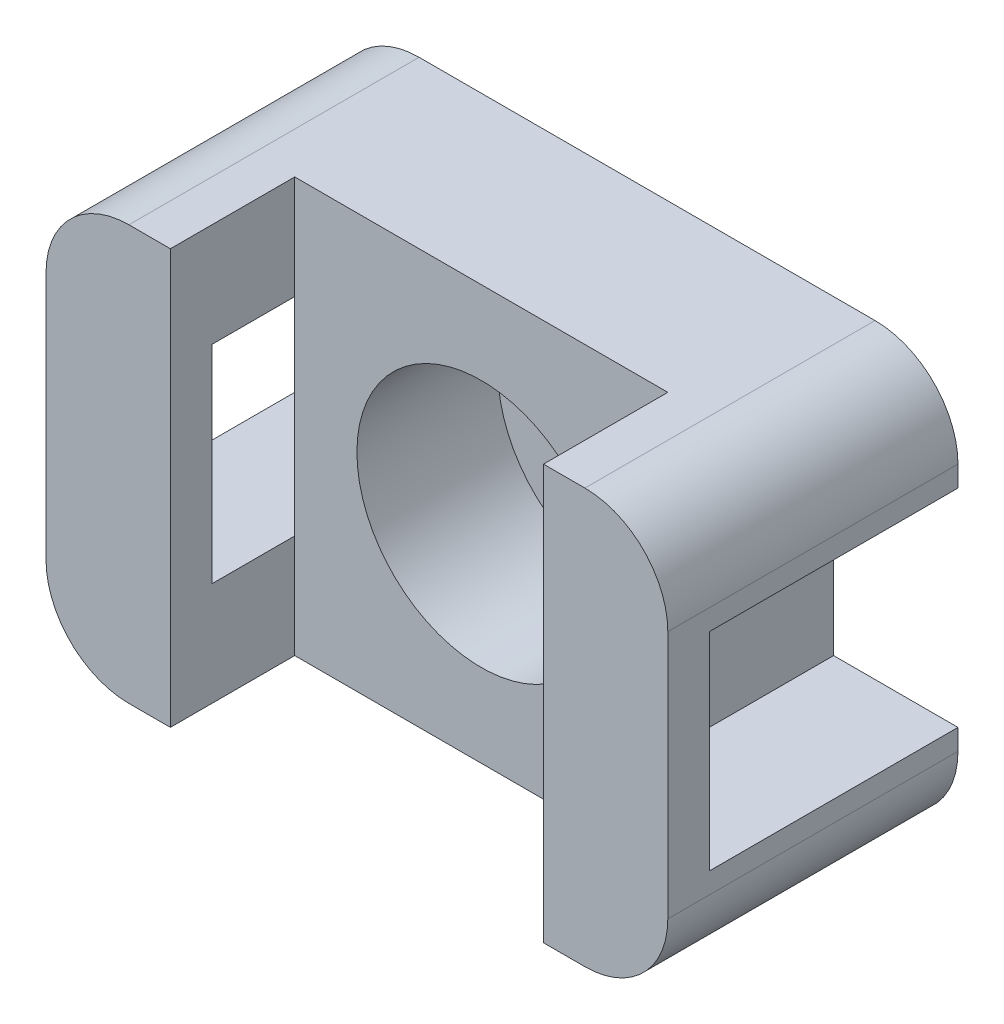
from build123d import *

# Parameters (mm, degrees)
SKETCH1_W                                            = 15
SKETCH1_H                                            = 10
BOSS_EXTRUDE1_DEPTH                                  = 7
SKETCH2_W                                            = 9
SKETCH2_H                                            = 15.767491366
CUT_EXTRUDE1_DEPTH                                   = 3
SKETCH4_W                                            = 6
SKETCH4_H                                            = 5
CUT_EXTRUDE3_DEPTH                                   = 6
HOLE_SIZE_PER_SOCKET_HEAD_CAP_SCREW_TYPE_D           = 3.4
HOLE_SIZE_PER_SOCKET_HEAD_CAP_SCREW_TYPE_CBORE_D     = 6
HOLE_SIZE_PER_SOCKET_HEAD_CAP_SCREW_TYPE_CBORE_DEPTH = 3.4
FILLET1_R                                            = 2


with BuildPart() as part:
    # Sketch1 → Boss-Extrude1 (new body)
    with BuildSketch(Plane.XY):
        Rectangle(SKETCH1_W, SKETCH1_H)
    extrude(amount=BOSS_EXTRUDE1_DEPTH)

    # Sketch2 → Cut-Extrude1 (cut)
    with BuildSketch(Plane.XY.offset(7)):
        Rectangle(SKETCH2_W, SKETCH2_H)
    extrude(amount=-CUT_EXTRUDE1_DEPTH, mode=Mode.SUBTRACT)

    # Sketch4 → Cut-Extrude3 (cut)
    with BuildSketch(Plane(origin=(0, 0, 0), x_dir=(-1, 0, 0), z_dir=(0, 0, -1))):
        with Locations((-7.5, 0)):
            Rectangle(SKETCH4_W, SKETCH4_H)
        with Locations((7.5, 0)):
            Rectangle(SKETCH4_W, SKETCH4_H)
    extrude(amount=-CUT_EXTRUDE3_DEPTH, mode=Mode.SUBTRACT)

    # Hole size per socket head cap screw type 1 (through all)
    with Locations(Plane.XY.offset(4)):
        with Locations((0, 0)):
            CounterBoreHole(HOLE_SIZE_PER_SOCKET_HEAD_CAP_SCREW_TYPE_D / 2, HOLE_SIZE_PER_SOCKET_HEAD_CAP_SCREW_TYPE_CBORE_D / 2, HOLE_SIZE_PER_SOCKET_HEAD_CAP_SCREW_TYPE_CBORE_DEPTH)

    # Fillet1
    fillet1_edges = [part.edges().sort_by_distance(p)[0] for p in [
        (7.5, -5, 3.5),
        (-7.5, -5, 3.5),
        (-7.5, 5, 3.5),
        (7.5, 5, 3.5),
    ]]
    fillet(fillet1_edges, radius=FILLET1_R)


solid = part.part
